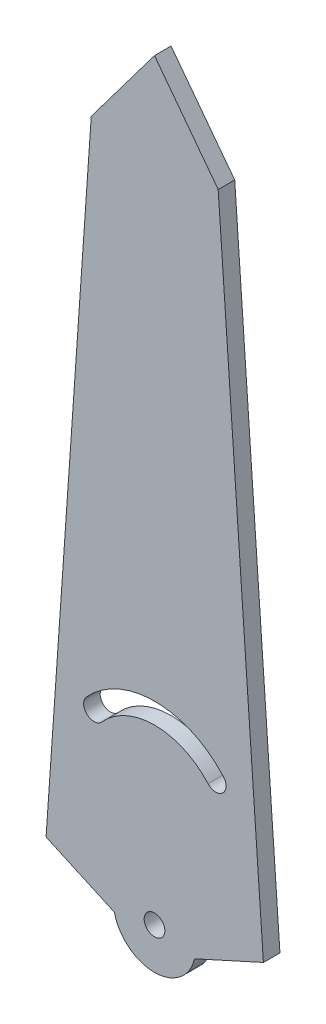
SolidWorks part; units mm, degrees
ref_plane "Front Plane" through (0, 0, 0) normal (0, 0, 1) x (1, 0, 0)
ref_plane "Top Plane" through (0, 0, 0) normal (0, 1, 0) x (1, 0, 0)
ref_plane "Right Plane" through (0, 0, 0) normal (1, 0, 0) x (0, 0, -1)
other "Configuration Table"
sketch "Sketch2" plane through (0, 0, 0) normal (0, 0, 1) x (1, 0, 0)
  line L1 (52.6614, 1194.6) -> (30.7927, 1507.337)
  line L2 (52.6614, 1194.6) -> (19.3758, 1179.501)
  line L3 (-52.4386, 1194.6) -> (-30.5699, 1507.337)
  line L4 (-52.4386, 1194.6) -> (-19.4017, 1179.6138)
  line L5 (0, 1548.0522) -> (-30.5699, 1507.337)
  line L6 (0, 1548.0522) -> (30.7927, 1507.337)
  arc A3 (-19.4017, 1179.6138) -> (19.3758, 1179.501) centre (0, 1184) ccw
  circle A6 centre (0, 1184) radius 5
  dimension "D2" = 105.1
  dimension "D3" = 110.4
  dimension "D4" = 8
  dimension "D6" = 110.4
  dimension "D7" = 74
  dimension "D8" = 147.1
extrude "Boss-Extrude1" add sketch "Sketch2" along normal blind 8
sketch "Sketch3" plane through (0, 0, 8) normal (0, 0, 1) x (1, 0, 0)
  line L0 (-47.7242, 1262.0188) -> (47.947, 1262.0188) construction
  line L1 (-30.5699, 1507.337) -> (-52.4386, 1194.6) construction
  line L2 (52.6614, 1194.6) -> (30.7927, 1507.337) construction
  arc A0 (-32.9948, 1262.8592) -> (33.3461, 1262.7142) centre (0.1114, 1233.389) cw
  arc A1 (-25.5255, 1256.2102) -> (26.3131, 1255.5594) centre (0.1114, 1233.389) cw
  arc A2 (-32.9948, 1262.8592) -> (-25.5255, 1256.2102) centre (-29.2601, 1259.5347) ccw
  arc A3 (25.8478, 1256.0979) -> (33.3461, 1262.7142) centre (29.597, 1259.4061) ccw
  arc A4 (-33.7242, 1262.0188) -> (33.947, 1262.0188) centre (0.1114, 1233.389) cw construction
  arc A5 (-26.0903, 1255.5594) -> (26.3131, 1255.5594) centre (0.1114, 1233.389) cw construction
  dimension "D3" = 10
extrude "Cut-Extrude1" cut sketch "Sketch3" against normal blind 10 contours A1 A3 A0 A2
